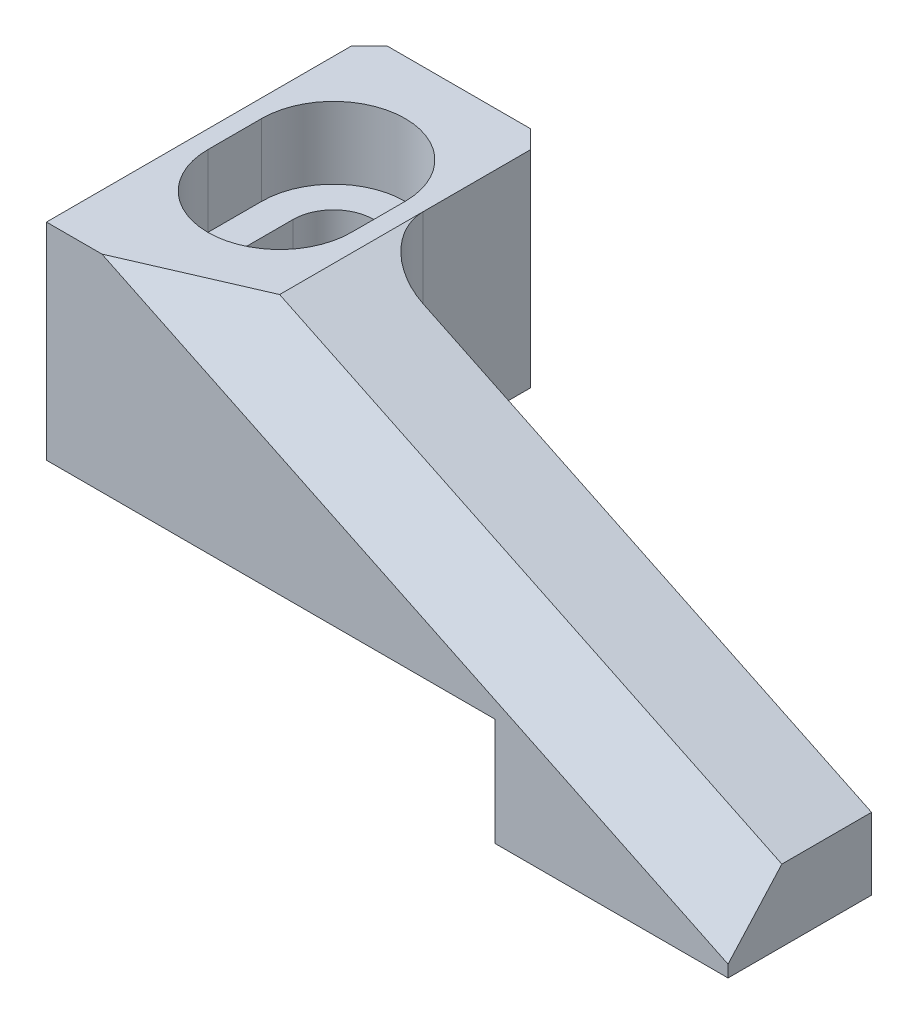
SolidWorks part; units mm, degrees
material "S45C"
ref_plane "Front Plane" through (0, 0, 0) normal (0, 0, 1) x (1, 0, 0)
ref_plane "Top Plane" through (0, 0, 0) normal (0, 1, 0) x (1, 0, 0)
ref_plane "Right Plane" through (0, 0, 0) normal (1, 0, 0) x (0, 0, -1)
sketch "Sketch1" plane through (0, 0, 0) normal (0, 0, 1) x (1, 0, 0)
  line L0 (0, 17.5) -> (0, 0)
  line L1 (0, 0) -> (38, 0)
  line L2 (38, 0) -> (38, 4)
  line L3 (38, 4) -> (10, 17.5)
  line L4 (10, 17.5) -> (0, 17.5)
  dimension "D1" = 10
  dimension "D2" = 38
  dimension "D3" = 4
  dimension "D4" = 17.5
extrude "Boss-Extrude1" add sketch "Sketch1" along normal blind 18
chamfer "Chamfer1" distance 3 distance2 3 1 edges at (24, 10.75, 18)
sketch "Sketch2" plane through (0, 17.5, 0) normal (0, 1, 0) x (1, 0, 0)
  line L0 (5, -10) -> (5, -7) construction
  line L1 (2.75, -10) -> (2.75, -7)
  line L2 (7.25, -10) -> (7.25, -7)
  line L3 (0, -18) -> (0, 0) construction
  line L4 (10, 0) -> (0, 0) construction
  arc A0 (2.75, -10) -> (7.25, -10) centre (5, -10) ccw
  arc A1 (7.25, -7) -> (2.75, -7) centre (5, -7) ccw
  point P2 (5, -8.5)
  dimension "D1" = 3
  dimension "D3" = 2.25
  dimension "D4" = 7
  dimension "D2" = 5
extrude "Cut-Extrude1" cut sketch "Sketch2" against normal blind 20
sketch "Sketch4" plane through (0, 17.5, 0) normal (0, 1, 0) x (1, 0, 0)
  line L0 (5, -7) -> (5, -10) construction
  line L1 (9, -7) -> (9, -10)
  line L2 (1, -7) -> (1, -10)
  arc A0 (9, -7) -> (1, -7) centre (5, -7) ccw
  arc A1 (1, -10) -> (9, -10) centre (5, -10) ccw
  point P4 (5, -8.5)
  dimension "D1" = 4
extrude "Cut-Extrude3" cut sketch "Sketch4" against normal blind 4
sketch "Sketch3" plane through (0, 0, 18) normal (0, 0, 1) x (1, 0, 0)
  line L1 (0, 0) -> (25, 0)
  line L2 (0, 0) -> (0, 6)
  line L3 (0, 6) -> (25, 6)
  line L4 (25, 0) -> (25, 6)
  dimension "D1" = 6
  dimension "D2" = 25
extrude "Cut-Extrude2" cut sketch "Sketch3" against normal through all
sketch "Sketch5" plane through (0, 17.5, 0) normal (0, 1, 0) x (-1, 0, 0)
  line L0 (-10, 15) -> (-10, 0) construction
  line L1 (-38, 0) -> (-10, 0)
  line L2 (-38, 0) -> (-38, 10)
  line L3 (-38, 10) -> (-10, 10)
  line L4 (-10, 0) -> (-10, 10)
  dimension "D1" = 10
extrude "Cut-Extrude4" cut sketch "Sketch5" against normal through all
fillet "Fillet1" radius 3 1 edges at (10, 11.75, 10)
chamfer "Chamfer2" distance 1 angle 45 2 edges at (0, 11.75, 0) (10, 11.75, 0)
